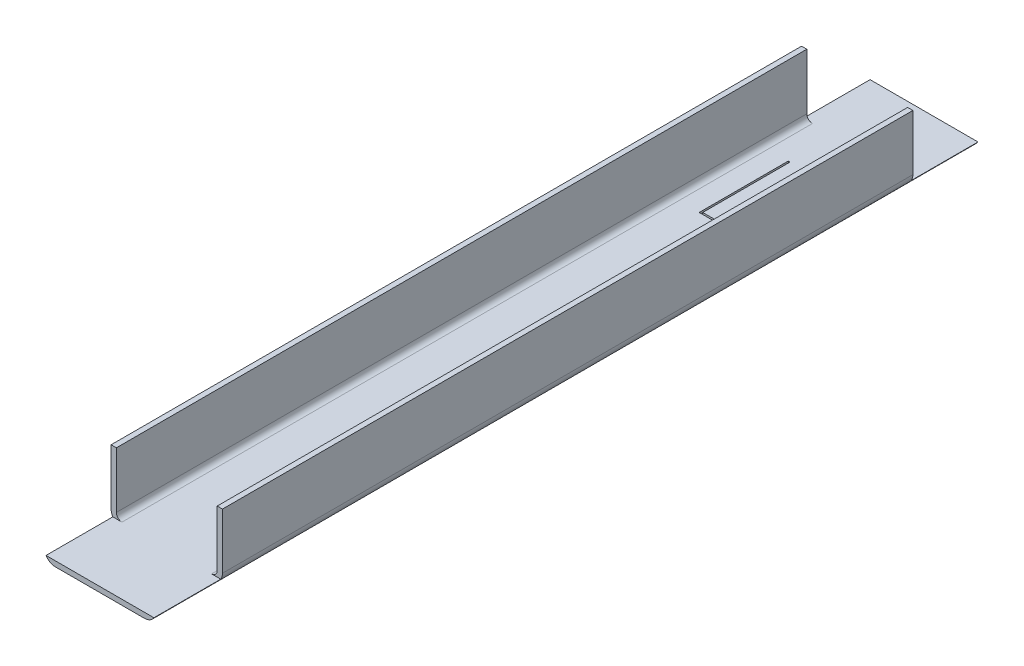
SolidWorks part; units mm, degrees
ref_plane "Front Plane" through (0, 0, 0) normal (0, 0, 1) x (1, 0, 0)
ref_plane "Top Plane" through (0, 0, 0) normal (0, 1, 0) x (1, 0, 0)
ref_plane "Right Plane" through (0, 0, 0) normal (1, 0, 0) x (0, 0, -1)
sketch "Sketch1" plane through (0, 0, 0) normal (0, 0, 1) x (1, 0, 0)
  line L0 (30.25, 3.1) -> (30.25, 19.05)
  line L1 (3.2, 0) -> (28.55, 0)
  line L2 (0, 3.2) -> (0, 19.05)
  line L3 (3.1, 1.5) -> (28.65, 1.5)
  line L4 (31.75, 3.2) -> (31.75, 19.05)
  line L5 (1.5, 3.1) -> (1.5, 19.05)
  line L6 (1.5, 19.05) -> (0, 19.05)
  line L7 (31.75, 19.05) -> (30.25, 19.05)
  line L8 (1.5, 1.5) -> (30.25, 1.5) construction
  line L9 (1.5, 1.5) -> (1.5, 19.05) construction
  line L10 (30.25, 1.5) -> (30.25, 19.05) construction
  line L11 (31.75, 0) -> (31.75, 19.05) construction
  line L12 (0, 0) -> (31.75, 0) construction
  line L13 (0, 0) -> (0, 19.05) construction
  arc A0 (3.1, 1.5) -> (1.5, 3.1) centre (3.1, 3.1) cw
  arc A1 (28.65, 1.5) -> (30.25, 3.1) centre (28.65, 3.1) ccw
  arc A2 (31.75, 3.2) -> (28.55, 0) centre (28.55, 3.2) cw
  arc A3 (0, 3.2) -> (3.2, 0) centre (3.2, 3.2) ccw
  dimension "D4" = 1.6
  dimension "D5" = 1.6
  dimension "D6" = 3.2
  dimension "D7" = 3.2
  dimension "D2" = 31.75
  dimension "D3" = 1.5
extrude "Boss-Extrude1" add sketch "Sketch1" along normal blind 234.95
sketch "Sketch2" plane through (0, 0, 0) normal (1, 0, 0) x (0, 0, -1)
  line L0 (0, 3.2) -> (0, 19.05) construction
  line L1 (0, 1.5) -> (0, 19.05)
  line L2 (-234.95, 3.2) -> (-234.95, 19.05) construction
  line L3 (-234.95, 1.5) -> (-234.95, 19.05)
  line L4 (-234.95, 1.5) -> (0, 1.5) construction
  line L5 (-234.95, 1.5) -> (-215.9, 1.5)
  line L6 (-215.9, 1.5) -> (-215.9, 19.05)
  line L7 (-234.95, 3.2) -> (-234.95, 19.05) construction
  line L8 (-215.9, 3.2) -> (-215.9, 19.05) construction
  line L9 (-19.05, 1.5) -> (-19.05, 19.05)
  line L10 (0, 3.2) -> (0, 19.05) construction
  line L11 (-19.05, 3.2) -> (-19.05, 19.05) construction
  line L12 (-19.05, 1.5) -> (0, 1.5)
  line L13 (-19.05, 19.05) -> (0, 19.05)
  line L14 (-234.95, 19.05) -> (-215.9, 19.05)
  dimension "D1" = 19.05
  dimension "D2" = 19.05
extrude "Cut-Extrude1" cut sketch "Sketch2" along normal through all
sketch "Sketch3" plane through (0, 0, 0) normal (0, 1, 0) x (1, 0, 0)
  line L0 (31.2611, -234.95) -> (0.4889, -234.95) construction
  line L1 (22.8218, -57.15) -> (8.9282, -57.15)
  line L2 (9.4282, -31.75) -> (9.4282, -56.65)
  line L3 (22.3218, -56.65) -> (9.4282, -56.65)
  line L4 (15.875, 0) -> (15.875, -77.307) construction
  line L5 (31.2611, 0) -> (0.4889, 0) construction
  line L6 (8.9282, -31.75) -> (8.9282, -57.15)
  line L7 (22.8218, -31.75) -> (22.8218, -57.15)
  line L8 (22.3218, -31.75) -> (22.3218, -56.65)
  line L9 (9.4282, -31.75) -> (8.9282, -31.75)
  line L10 (22.8218, -31.75) -> (22.3218, -31.75)
  point P0 (31.2611, -57.15)
  point P1 (0.4889, -57.15)
  point P2 (31.2611, -31.75)
  point P3 (0.4889, -31.75)
  dimension "D2" = 203.2
  dimension "D1" = 0.5
extrude "Cut-Extrude2" cut sketch "Sketch3" along normal through all
